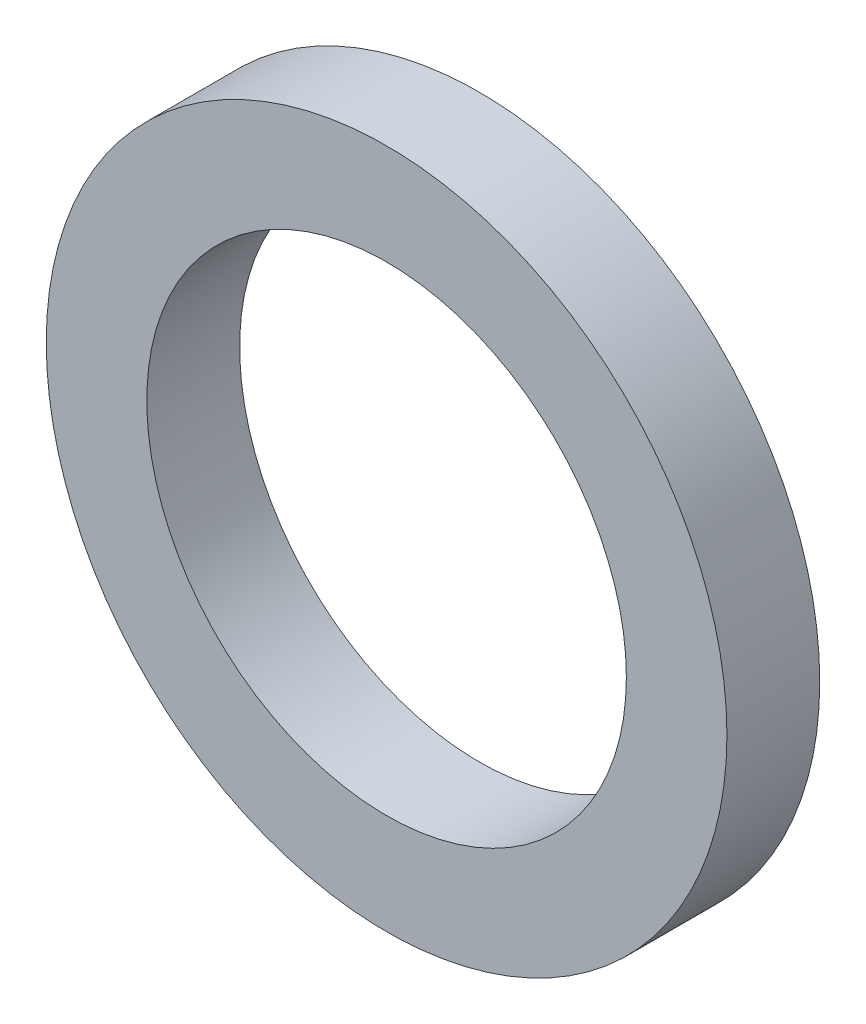
SolidWorks part; units mm, degrees
ref_plane "前视基准面" through (0, 0, 0) normal (0, 0, 1) x (1, 0, 0)
ref_plane "上视基准面" through (0, 0, 0) normal (0, 1, 0) x (1, 0, 0)
ref_plane "右视基准面" through (0, 0, 0) normal (1, 0, 0) x (0, 0, -1)
other "Configuration Table"
sketch "草图1" plane through (0, 0, 0) normal (0, 0, 1) x (1, 0, 0)
  circle A0 centre (0, 0) radius 11
  circle A1 centre (0, 0) radius 7.75
  dimension "D1" = 22
  dimension "D2" = 15.5
extrude "凸台-拉伸1" add sketch "草图1" along normal blind 3
